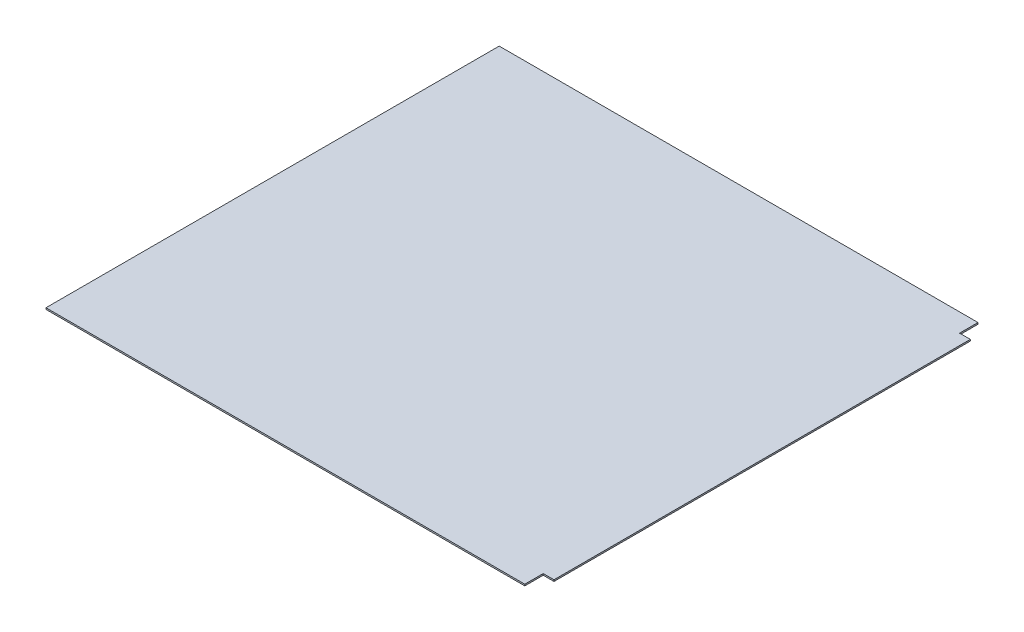
SolidWorks part; units mm, degrees
material "Q235"
ref_plane "Front Plane" through (0, 0, 0) normal (0, 0, 1) x (1, 0, 0)
ref_plane "Top Plane" through (0, 0, 0) normal (0, 1, 0) x (1, 0, 0)
ref_plane "Right Plane" through (0, 0, 0) normal (1, 0, 0) x (0, 0, -1)
sketch "Sketch1" plane through (0, 0, 0) normal (0, 1, 0) x (1, 0, 0)
  line L0 (-956, 0) -> (0, 0) construction
  line L5 (-21, -406.5) -> (0, -406.5)
  line L7 (-956, -442.5) -> (-956, 442.5)
  line L8 (-956, 442.5) -> (-21, 442.5)
  line L11 (-21, -406.5) -> (-21, -442.5)
  line L12 (-956, -442.5) -> (-21, -442.5)
  line L20 (-21, 406.5) -> (-21, 442.5)
  line L40 (-21, 406.5) -> (0, 406.5)
  line L41 (0, 406.5) -> (0, -406.5)
  point P0 (0, 0)
  point P13 (20.0634, -406.5)
  point P34 (20.0634, 406.5)
  dimension "D1" = 442.5
  dimension "D2" = 935
  dimension "D3" = 21
  dimension "D4" = 36
extrude "Boss-Extrude1" add sketch "Sketch1" along normal blind 3
